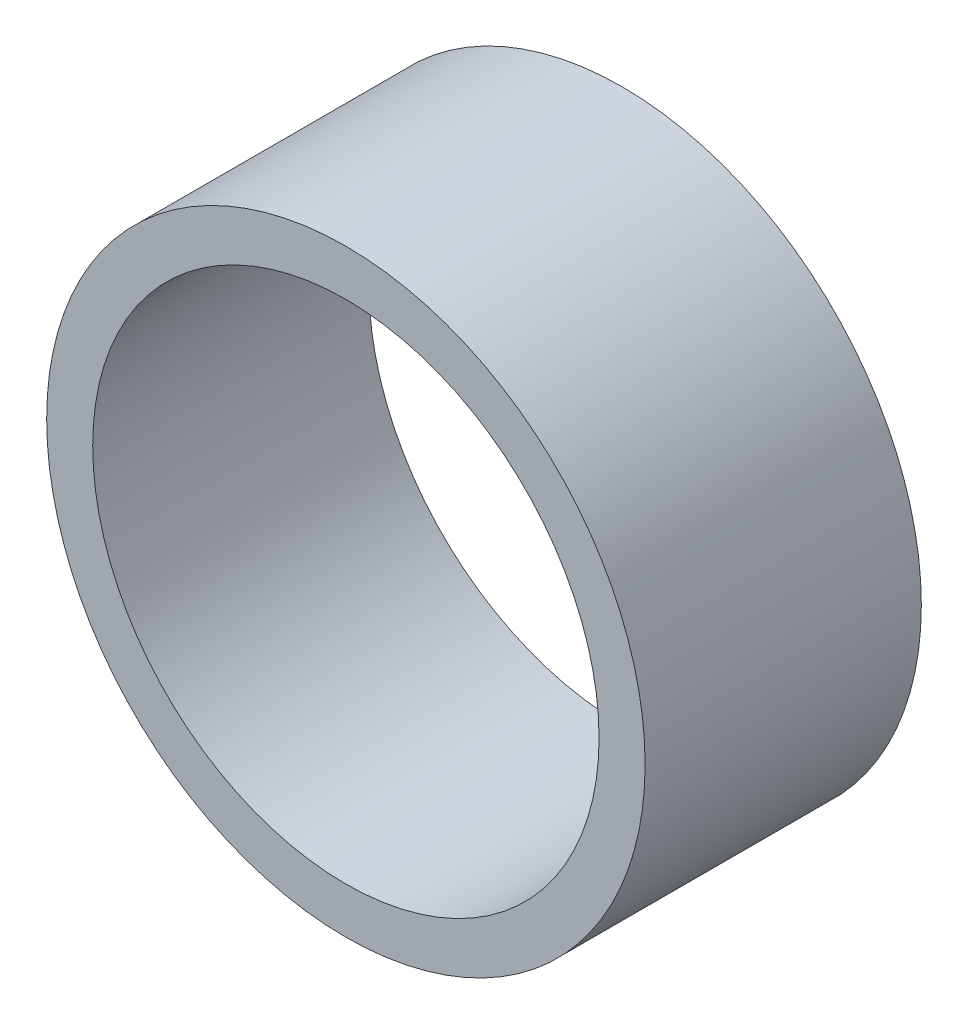
SolidWorks part; units mm, degrees
ref_plane "Front Plane" through (0, 0, 0) normal (0, 0, 1) x (1, 0, 0)
ref_plane "Top Plane" through (0, 0, 0) normal (0, 1, 0) x (1, 0, 0)
ref_plane "Right Plane" through (0, 0, 0) normal (1, 0, 0) x (0, 0, -1)
other "Configuration Table"
sketch "Sketch1" plane through (0, 0, 0) normal (0, 0, 1) x (1, 0, 0)
  circle A0 centre (0, 0) radius 27.5
  circle A1 centre (0, 0) radius 32.5
  dimension "D1" = 55
  dimension "D2" = 65
extrude "Boss-Extrude1" add sketch "Sketch1" along normal blind 30
